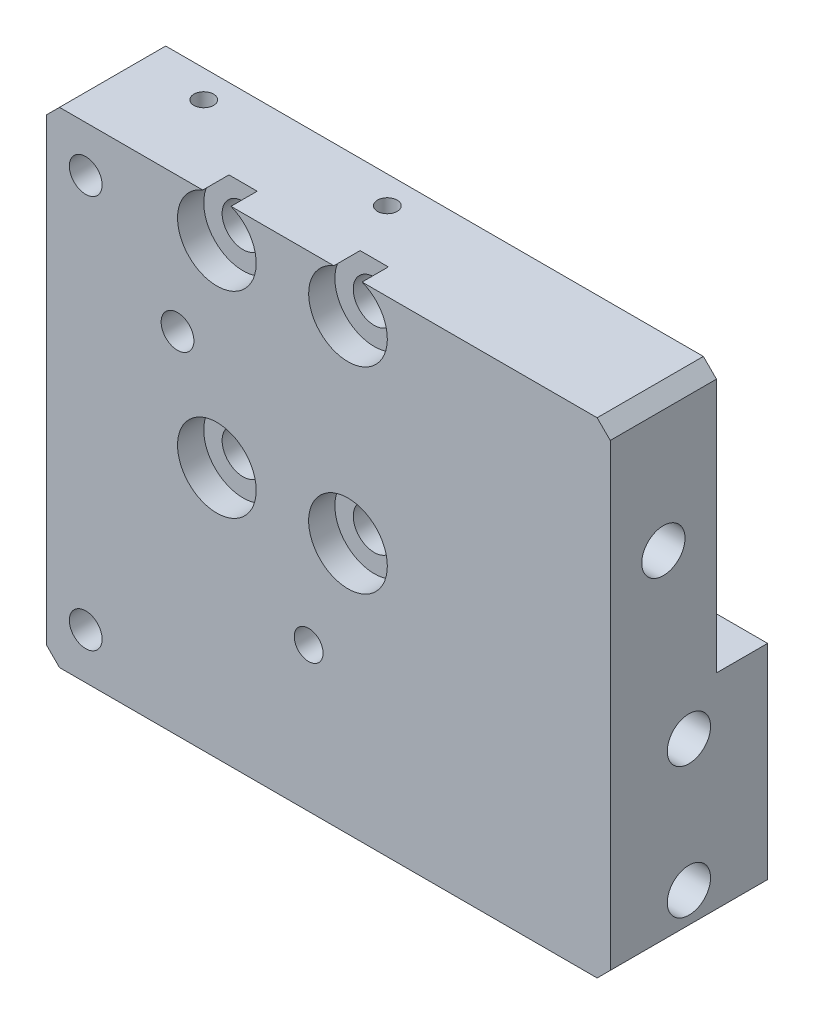
from build123d import *

# Parameters (mm, degrees)
SKETCH_1_W              = 40
SKETCH_1_H              = 27
EXTRUDE_1_DEPTH         = 6
SKETCH_2_R              = 1.1
CUT_EXTRUDE_1_DEPTH     = 10
MOVE_FACE_1_BY          = 10
SKETCH_3_W              = 3.9
SKETCH_3_H              = 20.4
CUT_EXTRUDE_2_DEPTH     = 63
HOLE_WIZARD_3_2_3_2_1_D = 3.2
MOVE_FACE_3_BY          = 3
HOLE_WIZARD_M4_2_D      = 3.3
HOLE_WIZARD_M4_2_DEPTH  = 11.5
HOLE_WIZARD_M4_2_TIP    = 0.991420021
SKETCH_16_R             = 3
CUT_EXTRUDE_3_DEPTH     = 2
HOLE_WIZARD_M3_1_D      = 2.5
HOLE_WIZARD_M3_1_DEPTH  = 8.5
HOLE_WIZARD_M3_1_TIP    = 0.751075774
CHAMFER_1_SIZE          = 1
SKETCH_20_R             = 0.75
CUT_EXTRUDE_4_DEPTH     = 66
PATTERN_LINEAR_1_COUNT  = 2
PATTERN_LINEAR_1_PITCH  = 14
HOLE_WIZARD_M3_2_D      = 2.5
HOLE_WIZARD_M3_3_D      = 2.5
HOLE_WIZARD_M3_3_DEPTH  = 8.5
HOLE_WIZARD_M3_3_TIP    = 0.751075774
HOLE_WIZARD_M4_3_D      = 3.3
HOLE_WIZARD_M4_3_DEPTH  = 11.5
HOLE_WIZARD_M4_3_TIP    = 0.991420021


with BuildPart() as part:
    # 草图1 → 凸台-拉伸1 (new, symmetric)
    with BuildSketch(Plane.XY):
        Rectangle(SKETCH_1_W, SKETCH_1_H)
    extrude(amount=EXTRUDE_1_DEPTH, both=True)

    # 草图2 → 切除-拉伸1 (cut)
    with BuildSketch(Plane.XY.offset(6)):
        with Locations((0, -2.5)):
            Circle(SKETCH_2_R)
    extrude(amount=-CUT_EXTRUDE_1_DEPTH, mode=Mode.SUBTRACT)

    # Move Face 1: a face moved outward by 10.0
    extrude(part.faces().sort_by_distance((0, 13.5, 0))[0], amount=MOVE_FACE_1_BY, dir=(0, 1, 0))

    # 草图3 → 切除-拉伸2 (cut)
    with BuildSketch(Plane(origin=(20, 0, 0), x_dir=(0, 0, -1), z_dir=(1, 0, 0))):
        with Locations((4.05, 13.3)):
            Rectangle(SKETCH_3_W, SKETCH_3_H)
    extrude(amount=-CUT_EXTRUDE_2_DEPTH, mode=Mode.SUBTRACT)

    # Ø3.2 (3.2) 直径孔1 (through all)
    with Locations(Plane.XY.offset(6)):
        with Locations((3, 20.7), (-7, 20.7), (-7, 5.7), (3, 5.7)):
            Hole(HOLE_WIZARD_3_2_3_2_1_D / 2)

    # Move Face 3: a face moved outward by 3.0
    extrude(part.faces().sort_by_distance((20, 3.188047415, 0.884145538))[0], amount=MOVE_FACE_3_BY, dir=(1, 0, 0))

    # M4 螺纹孔2
    with Locations(Plane(origin=(23, 0, 0), x_dir=(0, 0, -1), z_dir=(1, 0, 0))):
        with Locations((0, -0.2), (0, -10.2)):
            Hole(HOLE_WIZARD_M4_2_D / 2, depth=HOLE_WIZARD_M4_2_DEPTH)
            with Locations((0, 0, -(HOLE_WIZARD_M4_2_DEPTH + HOLE_WIZARD_M4_2_TIP / 2))):  # 118° drill point
                Cone(0, HOLE_WIZARD_M4_2_D / 2, HOLE_WIZARD_M4_2_TIP, mode=Mode.SUBTRACT)

    # 草图16 → 切除-拉伸3 (cut)
    with BuildSketch(Plane.XY.offset(6)):
        with Locations((-7, 20.7)):
            Circle(SKETCH_16_R)
        with Locations((3, 20.7)):
            Circle(SKETCH_16_R)
        with Locations((-7, 5.7)):
            Circle(SKETCH_16_R)
        with Locations((3, 5.7)):
            Circle(SKETCH_16_R)
    extrude(amount=-CUT_EXTRUDE_3_DEPTH, mode=Mode.SUBTRACT)

    # M3 螺纹孔1
    with Locations(Plane.XY.offset(6)):
        with Locations((-17, 20), (-17, -10)):
            Hole(HOLE_WIZARD_M3_1_D / 2, depth=HOLE_WIZARD_M3_1_DEPTH)
            with Locations((0, 0, -(HOLE_WIZARD_M3_1_DEPTH + HOLE_WIZARD_M3_1_TIP / 2))):  # 118° drill point
                Cone(0, HOLE_WIZARD_M3_1_D / 2, HOLE_WIZARD_M3_1_TIP, mode=Mode.SUBTRACT)

    # 倒角1
    chamfer_1_edges = [part.edges().sort_by_distance(p)[0] for p in [
        (23, -13.5, 0),
        (-20, -13.5, 0),
        (-20, 23.5, 1.95),
        (23, 23.5, 1.95),
    ]]
    chamfer(chamfer_1_edges, length=CHAMFER_1_SIZE)

    # 草图20 → 切除-拉伸4 (cut)
    with BuildSketch(Plane.XZ.offset(13.5)):
        with Locations(Location((0, 0, 0), (0, 0, 270))):
            Circle(SKETCH_20_R)
    cut_extrude_4 = extrude(amount=-CUT_EXTRUDE_4_DEPTH, mode=Mode.SUBTRACT)

    # 阵列(线性)1: 切除-拉伸4 ×2
    with Locations(*[(-i * PATTERN_LINEAR_1_PITCH, 0, 0) for i in range(1, PATTERN_LINEAR_1_COUNT)]):
        add(cut_extrude_4, mode=Mode.SUBTRACT)

    # M3 螺纹孔2 (through all)
    with Locations(Plane.XY.offset(6)):
        with Locations((-10, 13.2)):
            Hole(HOLE_WIZARD_M3_2_D / 2)

    # M3 螺纹孔3
    with Locations(Plane(origin=(0, -13.5, 0), x_dir=(-1, 0, 0), z_dir=(0, -1, 0))):
        with Locations((7.5, 0), (14, 0)):
            Hole(HOLE_WIZARD_M3_3_D / 2, depth=HOLE_WIZARD_M3_3_DEPTH)
            with Locations((0, 0, -(HOLE_WIZARD_M3_3_DEPTH + HOLE_WIZARD_M3_3_TIP / 2))):  # 118° drill point
                Cone(0, HOLE_WIZARD_M3_3_D / 2, HOLE_WIZARD_M3_3_TIP, mode=Mode.SUBTRACT)

    # M4 螺纹孔3
    with Locations(Plane(origin=(23, 0, 0), x_dir=(0, 0, -1), z_dir=(1, 0, 0))):
        with Locations((-1.95, 13.2)):
            Hole(HOLE_WIZARD_M4_3_D / 2, depth=HOLE_WIZARD_M4_3_DEPTH)
            with Locations((0, 0, -(HOLE_WIZARD_M4_3_DEPTH + HOLE_WIZARD_M4_3_TIP / 2))):  # 118° drill point
                Cone(0, HOLE_WIZARD_M4_3_D / 2, HOLE_WIZARD_M4_3_TIP, mode=Mode.SUBTRACT)


solid = part.part
